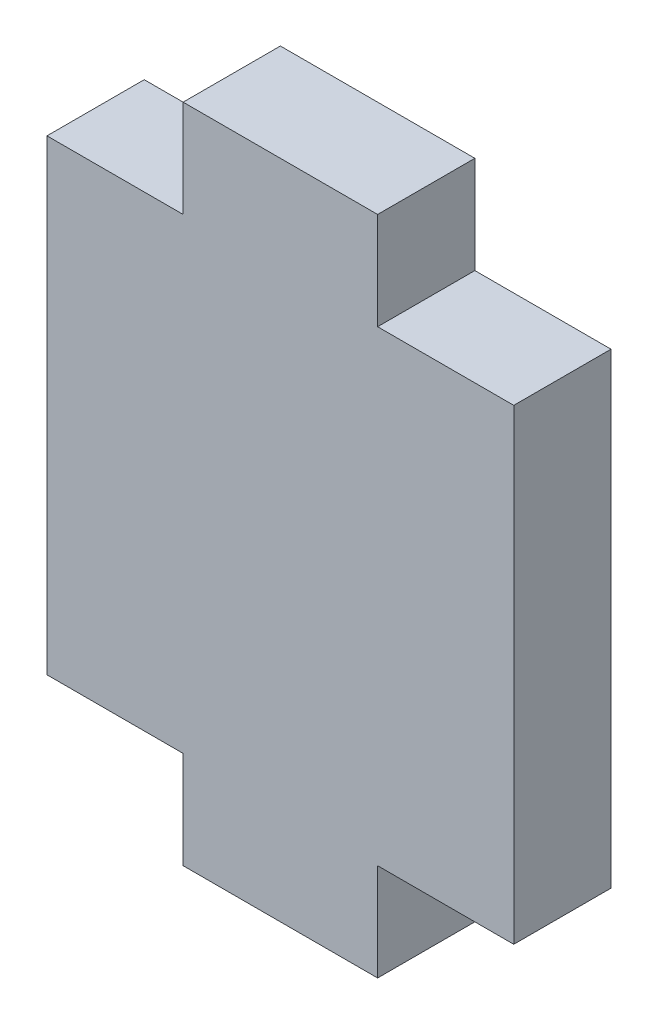
SolidWorks part; units mm, degrees
ref_plane "Front Plane" through (0, 0, 0) normal (0, 0, 1) x (1, 0, 0)
ref_plane "Top Plane" through (0, 0, 0) normal (0, 1, 0) x (1, 0, 0)
ref_plane "Right Plane" through (0, 0, 0) normal (1, 0, 0) x (0, 0, -1)
sketch "Sketch1" plane through (0, 0, 0) normal (0, 0, 1) x (1, 0, 0)
  line L1 (-24, 34) -> (24, 34)
  line L2 (-24, 34) -> (-24, -34)
  line L3 (-24, -34) -> (24, -34)
  line L4 (24, 34) -> (24, -34)
  line L5 (-24, 34) -> (24, -34) construction
  line L6 (-24, -34) -> (24, 34) construction
  point P0 (0, 0)
  dimension "D1" = 48
  dimension "D2" = 68
extrude "Boss-Extrude1" add sketch "Sketch1" along normal blind 10
sketch "Sketch2" plane through (0, 0, 10) normal (0, 0, 1) x (1, 0, 0)
  line L0 (-24, 0) -> (24, 0) construction
  line L5 (-24, 34) -> (-16.9412, 24) construction
  line L6 (-24, 34) -> (-24, -34) construction
  line L7 (-38, 44) -> (-10, 44)
  line L8 (-38, 44) -> (-38, 24)
  line L9 (-38, 24) -> (-10, 24)
  line L10 (-10, 44) -> (-10, 24)
  line L11 (-38, 44) -> (-10, 24) construction
  line L12 (-38, 24) -> (-10, 44) construction
  line L17 (24, -34) -> (24, 34) construction
  line L18 (0, 34) -> (0, -34) construction
  line L19 (24, 34) -> (-24, 34) construction
  line L20 (-24, -34) -> (24, -34) construction
  line L21 (38, 24) -> (10, 44) construction
  line L22 (38, 44) -> (10, 24) construction
  line L23 (24, 34) -> (16.9412, 24) construction
  line L24 (10, 44) -> (10, 24)
  line L25 (38, 24) -> (10, 24)
  line L26 (38, 44) -> (38, 24)
  line L27 (38, 44) -> (10, 44)
  line L28 (38, -44) -> (10, -44)
  line L29 (10, -44) -> (10, -24)
  line L30 (24, -34) -> (16.9412, -24) construction
  line L31 (38, -44) -> (10, -24) construction
  line L32 (38, -24) -> (10, -44) construction
  line L33 (38, -44) -> (38, -24)
  line L34 (38, -24) -> (10, -24)
  line L35 (-38, -24) -> (-10, -44) construction
  line L36 (-38, -44) -> (-10, -24) construction
  line L37 (-24, -34) -> (-16.9412, -24) construction
  line L38 (-10, -44) -> (-10, -24)
  line L39 (-38, -24) -> (-10, -24)
  line L40 (-38, -44) -> (-38, -24)
  line L41 (-38, -44) -> (-10, -44)
  point P0 (0, 0)
  dimension "D1" = 20
  dimension "D2" = 28
  dimension "D3" = 20
extrude "Cut-Extrude1" cut sketch "Sketch2" against normal blind 10
